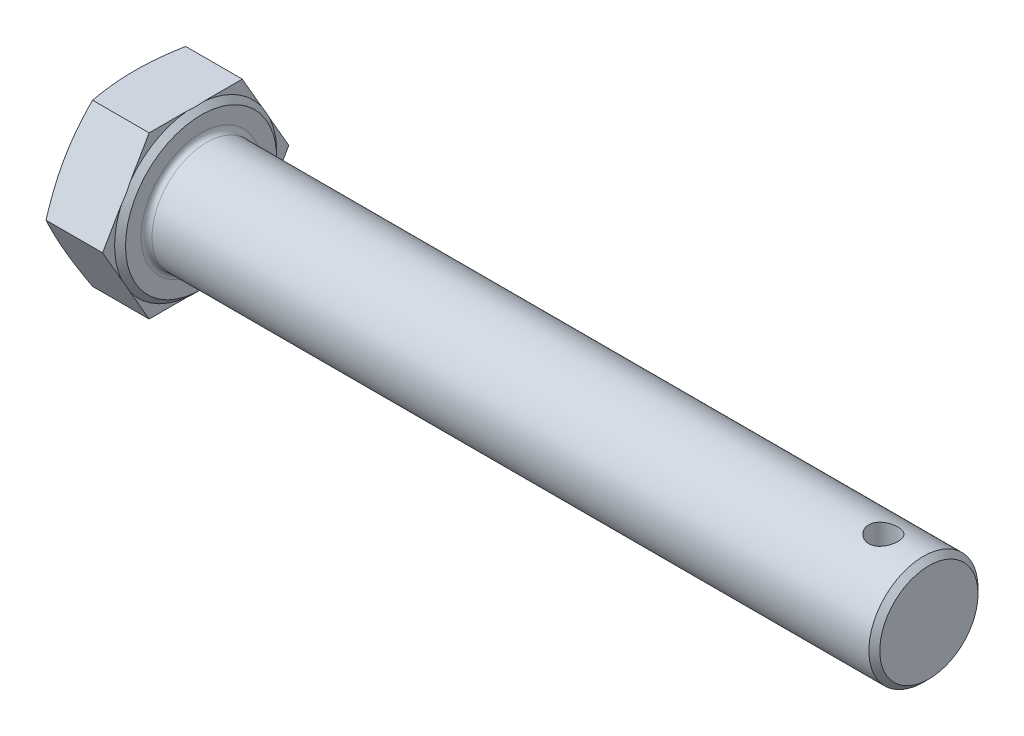
from build123d import *

# Parameters (mm, degrees)
BASEHEAD_DEPTH  = 7.32
SKETCH5_R       = 6
BASEBODY_DEPTH  = 80
CHAMFER1_SIZE   = 0.6
HOLE_DEPTH      = 89.363764774
HOLE_DEPTH_BACK = 89.363764774
SKETCH6_R       = 1.6
HEADFILLET_R    = 0.6


with BuildPart() as part:
    # Sketch2 → BaseHead (new body)
    with BuildSketch(Plane(origin=(0, 0, 0), x_dir=(0, 0, -1), z_dir=(1, 0, 0))):
        Polygon((10.236420273, 0), (5.118210136, 8.865), (-5.118210136, 8.865), (-10.236420273, 0), (-5.118210136, -8.865), (5.118210136, -8.865), align=None)
    extrude(amount=BASEHEAD_DEPTH)

    # Sketch3 → BearingFace (revolve, cut)
    with BuildSketch(Plane(origin=(0, 0, 0), x_dir=(1, 0, 0), z_dir=(0, 1, 0)), mode=Mode.PRIVATE) as bearingface_sk:
        Polygon((7.32, 10.236420273), (7.32, 8.315), (6.72, 8.915), (6.72, 10.236420273), align=None)
    revolve(bearingface_sk.sketch.rotate(Axis((-0.957090588, 0, 0), (1, 0, 0)), 180), axis=Axis((-0.957090588, 0, 0), (1, 0, 0)), mode=Mode.SUBTRACT)

    # Sketch4 → HeadChamfer (revolve, cut)
    with BuildSketch(Plane(origin=(0, 0, 0), x_dir=(1, 0, 0), z_dir=(0, 1, 0))):
        Polygon((0, 10.236420273), (0.499156158, 10.236420273), (0, 8.865), align=None)
    revolve(axis=Axis((-0.493528746, 0, 0), (1, 0, 0)), mode=Mode.SUBTRACT)

    # Sketch5 → BaseBody (add)
    with BuildSketch(Plane(origin=(7.32, 0, 0), x_dir=(0, 0, -1), z_dir=(1, 0, 0))):
        Circle(SKETCH5_R)
    extrude(amount=BASEBODY_DEPTH)

    # Chamfer1
    chamfer1_edges = [part.edges().sort_by_distance(p)[0] for p in [
        (87.32, 0, 6),
    ]]
    chamfer(chamfer1_edges, length=CHAMFER1_SIZE)

    # Sketch6 → Hole (cut, two sides: drawn at the far end of the back side and taken through both)
    with BuildSketch(Plane(origin=(0, 0, 0), x_dir=(1, 0, 0), z_dir=(0, 1, 0)).offset(-HOLE_DEPTH_BACK)):
        with Locations(Location((82.32, 0, 0), (0, 0, 270))):
            Circle(SKETCH6_R)
    extrude(amount=HOLE_DEPTH + HOLE_DEPTH_BACK, mode=Mode.SUBTRACT)

    # HeadFillet
    headfillet_edges = [part.edges().sort_by_distance(p)[0] for p in [
        (7.32, 0, 6),
    ]]
    fillet(headfillet_edges, radius=HEADFILLET_R)


solid = part.part
